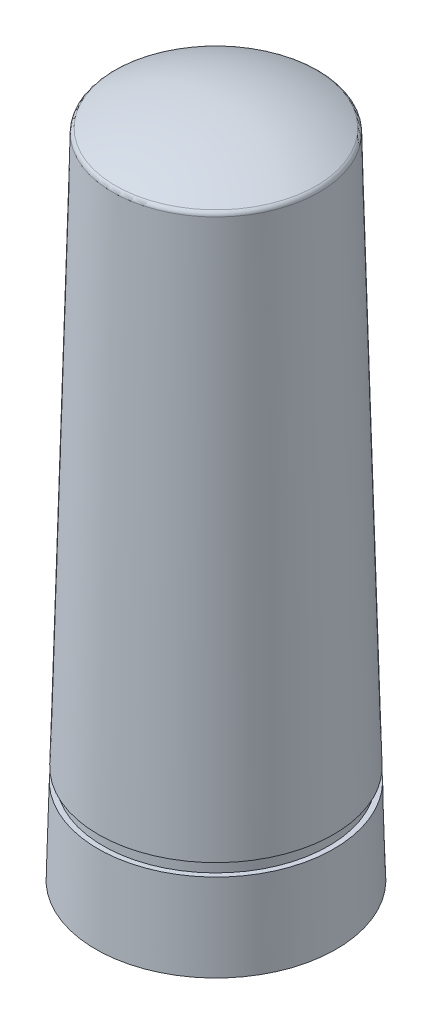
from build123d import *


with BuildPart() as part:
    # Sketch1 → Revolve1 (revolve)
    with BuildSketch(Plane.XY, mode=Mode.PRIVATE) as revolve1_sk:
        with BuildLine():
            Line((-4.9, 0), (-4.80754717, 3.5))
            Line((-4.80754717, 3.5), (-4.6, 3.5))
            Line((-4.6, 3.5), (-4.6, 4))
            Line((-4.6, 4), (-4.794339623, 4))
            Line((-4.794339623, 4), (-4.203177883, 26.379694424))
            ThreePointArc((-4.203177883, 26.379694424), (-4.171478034, 26.482572984), (-4.09103814, 26.554115293))
            ThreePointArc((-4.09103814, 26.554115293), (-2.09948154, 27.260450279), (0, 27.5))
            Line((0, 27.5), (0, 26.379694424))
            Line((0, 26.379694424), (-3.25, 26.379694424))
            Line((-3.25, 26.379694424), (-3.75, 1))
            Line((-3.75, 1), (-4, 1))
            Line((-4, 1), (-4, 0))
            Line((-4, 0), (-4.9, 0))
        make_face()
    revolve(revolve1_sk.sketch.rotate(Axis((0, 0, 0), (0, 1, 0)), 270), axis=Axis((0, 0, 0), (0, 1, 0)))


solid = part.part
